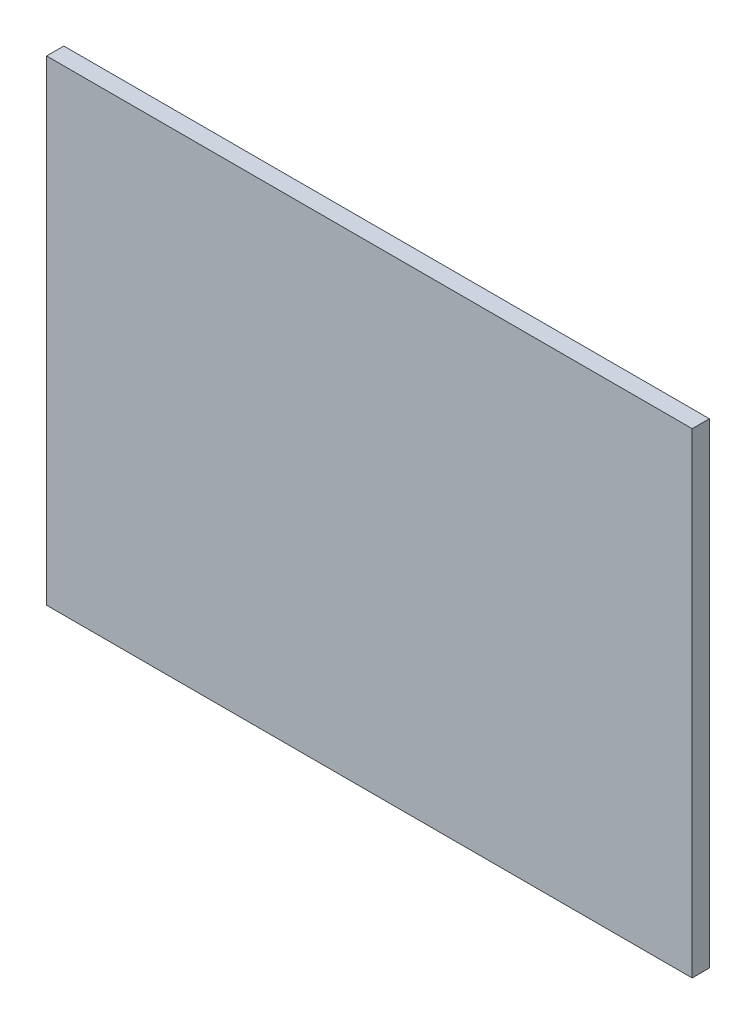
from build123d import *

# Parameters (mm, degrees)
SKETCH1_W           = 11.25
SKETCH1_H           = 8.29
BOSS_EXTRUDE1_DEPTH = 0.15


with BuildPart() as part:
    # Sketch1 → Boss-Extrude1 (new, symmetric)
    with BuildSketch(Plane.XY):
        Rectangle(SKETCH1_W, SKETCH1_H)
    extrude(amount=BOSS_EXTRUDE1_DEPTH, both=True)


solid = part.part
